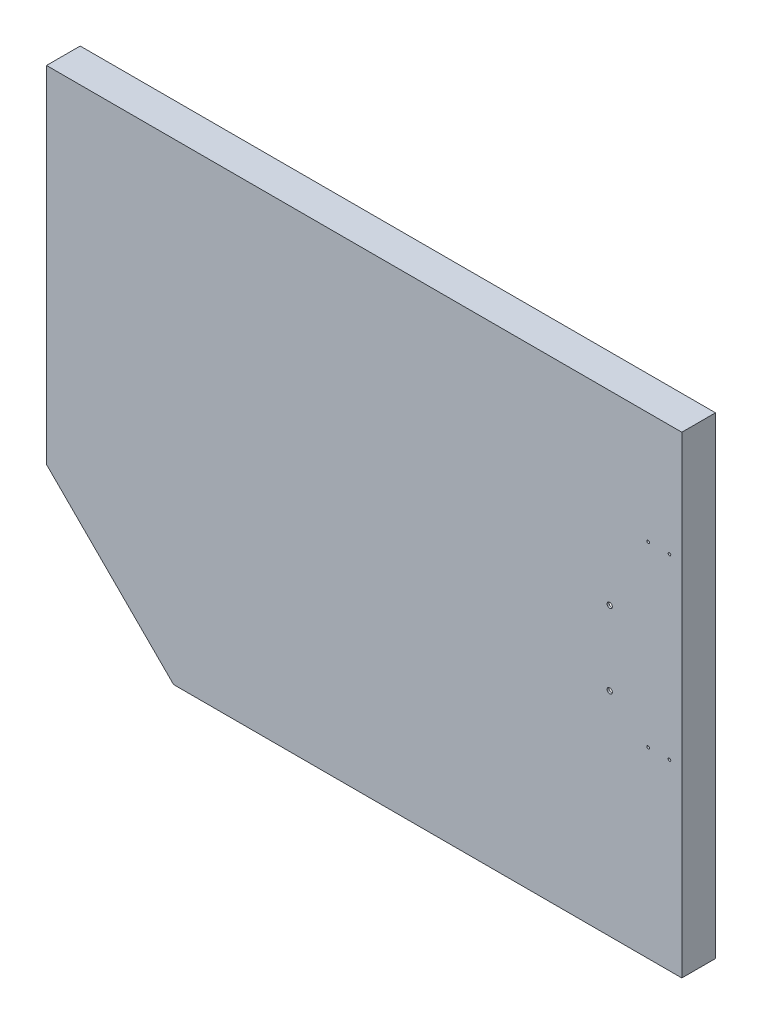
from build123d import *

# Parameters (mm, degrees)
EXTRUDE_1_DEPTH        = 50
EXTRUDE_1_2_DEPTH      = 3
CUT_EXTRUDE_1_REACH    = 640.784
SKETCH_3_R             = 4.1
HOLE_WIZARD_M8_1_D     = 6.8
HOLE_WIZARD_M8_1_DEPTH = 22.25
HOLE_WIZARD_M8_1_TIP   = 2.042926105
HOLE_WIZARD_M5_1_D     = 4.2


with BuildPart() as part:
    # 草图1 → Extrude 1 (new body)
    with BuildSketch(Plane.XY):
        Polygon((-500, 394), (-500, -150), (-300, -350), (500, -350), (500, 394), align=None)
        Polygon((-497, 391), (-497, -148.757359313), (-298.757359313, -347), (497, -347), (497, 391), align=None, mode=Mode.SUBTRACT)
    extrude(amount=EXTRUDE_1_DEPTH)

    # 草图2 → Extrude 1 2 (add)
    with BuildSketch(Plane.XY.offset(50)):
        Polygon((-500, -150), (-300, -350), (500, -350), (500, 394), (-500, 394), align=None)
    extrude(amount=EXTRUDE_1_2_DEPTH)

    # 草图3 → 切除-拉伸1 (cut, up to next)
    with BuildSketch(Plane.XY.offset(53), mode=Mode.PRIVATE) as cut_extrude_1_sk1:
        with Locations((386.5, 101.25)):
            Circle(SKETCH_3_R)
    cut_extrude_1_tool1 = extrude(cut_extrude_1_sk1.sketch, amount=-CUT_EXTRUDE_1_REACH, mode=Mode.PRIVATE) & part.part
    # 草图3 → 切除-拉伸1 (cut, up to next)
    with BuildSketch(Plane.XY.offset(53), mode=Mode.PRIVATE) as cut_extrude_1_sk2:
        with Locations((386.5, -15.25)):
            Circle(SKETCH_3_R)
    cut_extrude_1_tool2 = extrude(cut_extrude_1_sk2.sketch, amount=-CUT_EXTRUDE_1_REACH, mode=Mode.PRIVATE) & part.part
    add(cut_extrude_1_tool1.solids().sort_by_distance((386.5, 101.25, 53))[0], mode=Mode.SUBTRACT)
    add(cut_extrude_1_tool2.solids().sort_by_distance((386.5, -15.25, 53))[0], mode=Mode.SUBTRACT)

    # M8 螺纹孔1
    with Locations(Plane.ZY.offset(500)):
        with Locations((21, 284), (21, 254), (21, 54), (21, 24)):
            Hole(HOLE_WIZARD_M8_1_D / 2, depth=HOLE_WIZARD_M8_1_DEPTH)
            with Locations((0, 0, -(HOLE_WIZARD_M8_1_DEPTH + HOLE_WIZARD_M8_1_TIP / 2))):  # 118° drill point
                Cone(0, HOLE_WIZARD_M8_1_D / 2, HOLE_WIZARD_M8_1_TIP, mode=Mode.SUBTRACT)

    # M5 螺纹孔1 (through all)
    with Locations(Plane.XY.offset(53)):
        with Locations((447.014659804, -62), (480.514659804, -62), (447.014659804, 218), (480.514659804, 218)):
            Hole(HOLE_WIZARD_M5_1_D / 2)


solid = part.part
